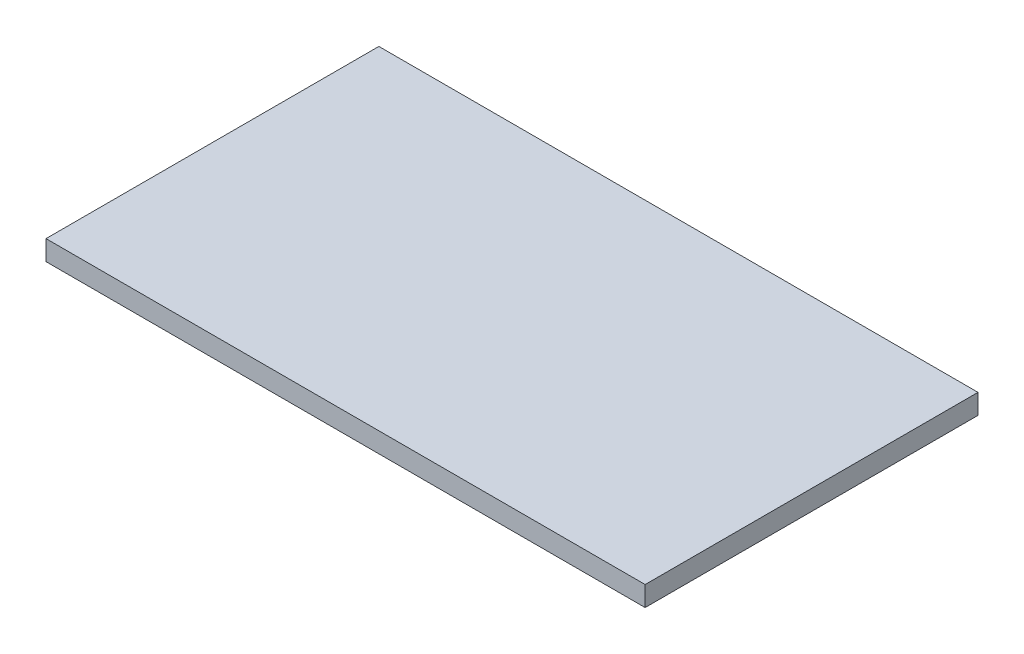
from build123d import *

# Parameters (mm, degrees)
SKETCH1_W           = 180
SKETCH1_H           = 100
BOSS_EXTRUDE1_DEPTH = 6


with BuildPart() as part:
    # Sketch1 → Boss-Extrude1 (new body)
    with BuildSketch(Plane(origin=(0, 0, 0), x_dir=(1, 0, 0), z_dir=(0, 1, 0))):
        Rectangle(SKETCH1_W, SKETCH1_H)
    extrude(amount=BOSS_EXTRUDE1_DEPTH)


solid = part.part
